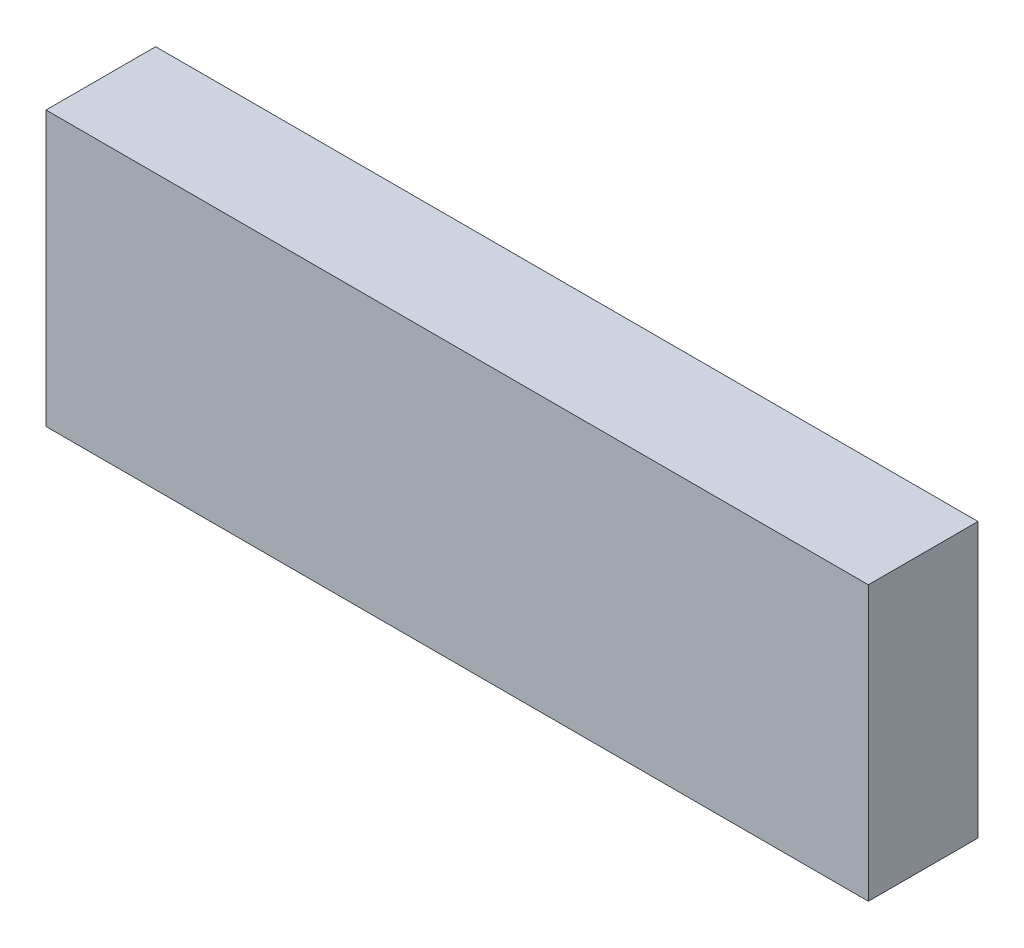
SolidWorks part; units mm, degrees
material "Q235"
ref_plane "Front Plane" through (0, 0, 0) normal (0, 0, 1) x (1, 0, 0)
ref_plane "Top Plane" through (0, 0, 0) normal (0, 1, 0) x (1, 0, 0)
ref_plane "Right Plane" through (0, 0, 0) normal (1, 0, 0) x (0, 0, -1)
sketch "Sketch1" plane through (0, 0, 0) normal (0, 0, 1) x (1, 0, 0)
  line L1 (-60, -20) -> (60, -20)
  line L2 (-60, -20) -> (-60, 20)
  line L3 (-60, 20) -> (60, 20)
  line L4 (60, -20) -> (60, 20)
  line L5 (-60, -20) -> (60, 20) construction
  line L6 (-60, 20) -> (60, -20) construction
  point P0 (0, 0)
  dimension "D1" = 120
  dimension "D2" = 40
extrude "Boss-Extrude1" add sketch "Sketch1" along normal mid plane 16
